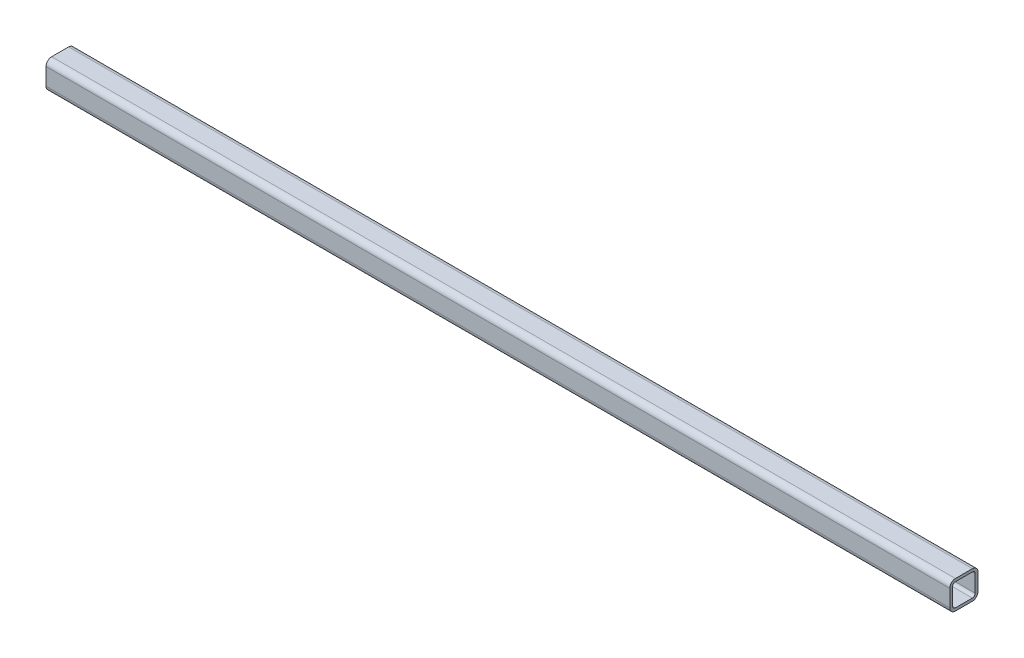
from build123d import *

# Parameters (mm, degrees)
SQUARE_TUBE_40_X_40_X_4_1_DEPTH = 1280


with BuildPart() as part:
    # Sketch1 → Square Tube 40 X 40 X 4(1) (new body)
    with BuildSketch(Plane.YZ.offset(-1000)):
        with BuildLine():
            Line((-12, -20), (12, -20))
            ThreePointArc((12, -20), (17.656854249, -17.656854249), (20, -12))
            Line((20, -12), (20, 12))
            ThreePointArc((20, 12), (17.656854249, 17.656854249), (12, 20))
            Line((12, 20), (-12, 20))
            ThreePointArc((-12, 20), (-17.656854249, 17.656854249), (-20, 12))
            Line((-20, 12), (-20, -12))
            ThreePointArc((-20, -12), (-17.656854249, -17.656854249), (-12, -20))
        make_face()
        with BuildLine():
            Line((-12, -16), (12, -16))
            ThreePointArc((12, -16), (14.828427125, -14.828427125), (16, -12))
            Line((16, -12), (16, 12))
            ThreePointArc((16, 12), (14.828427125, 14.828427125), (12, 16))
            Line((12, 16), (-12, 16))
            ThreePointArc((-12, 16), (-14.828427125, 14.828427125), (-16, 12))
            Line((-16, 12), (-16, -12))
            ThreePointArc((-16, -12), (-14.828427125, -14.828427125), (-12, -16))
        make_face(mode=Mode.SUBTRACT)
    extrude(amount=SQUARE_TUBE_40_X_40_X_4_1_DEPTH)


solid = part.part
